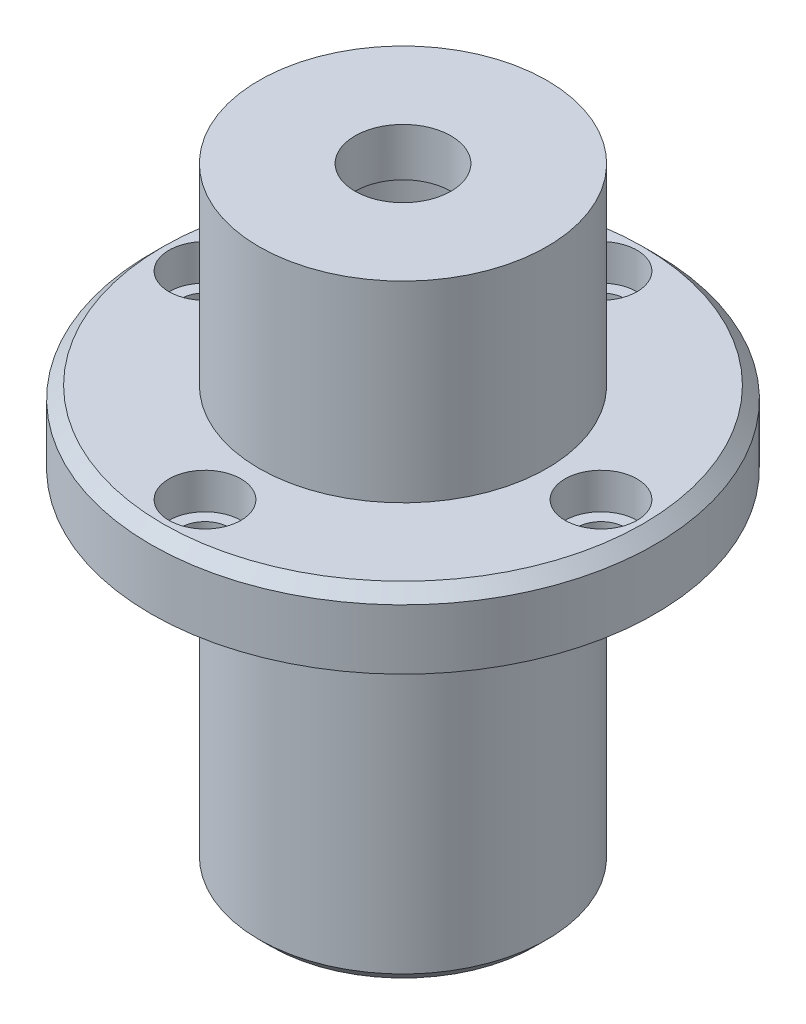
from build123d import *

# Parameters (mm, degrees)
SKETCH1_R           = 12
SKETCH1_R_2         = 4
BOSS_EXTRUDE1_DEPTH = 51
SKETCH2_R           = 8
CUT_EXTRUDE1_DEPTH  = 47
BOSS_EXTRUDE2_START = -6
SKETCH3_R           = 21
SKETCH3_R_2         = 12
BOSS_EXTRUDE2_DEPTH = 6
SKETCH4_R           = 2
CUT_EXTRUDE2_DEPTH  = 6
SKETCH5_R           = 3
CUT_EXTRUDE3_DEPTH  = 3
CIRPATTERN1_COUNT   = 4
CHAMFER1_SIZE       = 1


with BuildPart() as part:
    # Sketch1 → Boss-Extrude1 (new body)
    with BuildSketch(Plane(origin=(0, 0, 0), x_dir=(1, 0, 0), z_dir=(0, 1, 0))):
        with Locations(Location((0, 0, 0), (0, 0, 270))):
            Circle(SKETCH1_R)
        with Locations(Location((0, 0, 0), (0, 0, 270))):
            Circle(SKETCH1_R_2, mode=Mode.SUBTRACT)
    extrude(amount=BOSS_EXTRUDE1_DEPTH)

    # Sketch2 → Cut-Extrude1 (cut)
    with BuildSketch(Plane.XZ):
        with Locations(Location((0, 0, 0), (0, 0, 270))):
            Circle(SKETCH2_R)
    extrude(amount=-CUT_EXTRUDE1_DEPTH, mode=Mode.SUBTRACT)

    # Sketch3 → Boss-Extrude2 (add)
    with BuildSketch(Plane(origin=(0, 35, 0), x_dir=(-1, 0, 0), z_dir=(0, 1, 0)).offset(BOSS_EXTRUDE2_START)):
        with Locations(Location((0, 0, 0), (0, 0, 90))):
            Circle(SKETCH3_R)
        with Locations(Location((0, 0, 0), (0, 0, 90))):
            Circle(SKETCH3_R_2, mode=Mode.SUBTRACT)
    extrude(amount=BOSS_EXTRUDE2_DEPTH)

    # Sketch4 → Cut-Extrude2 (cut)
    with BuildSketch(Plane(origin=(0, 35, 0), x_dir=(1, 0, 0), z_dir=(0, 1, 0))):
        with Locations(Location((0, 16.5, 0), (0, 0, 270))):
            Circle(SKETCH4_R)
    cut_extrude2 = extrude(amount=-CUT_EXTRUDE2_DEPTH, mode=Mode.SUBTRACT)

    # Sketch5 → Cut-Extrude3 (cut)
    with BuildSketch(Plane(origin=(0, 35, 0), x_dir=(1, 0, 0), z_dir=(0, 1, 0))):
        with Locations(Location((0, 16.5, 0), (0, 0, 270))):
            Circle(SKETCH5_R)
    cut_extrude3 = extrude(amount=-CUT_EXTRUDE3_DEPTH, mode=Mode.SUBTRACT)

    # CirPattern1: Cut-Extrude2, Cut-Extrude3 ×4 about axis
    cirpattern1_axis = Axis((0, 0, 0), (0, 1, 0))
    add([cut_extrude2.rotate(cirpattern1_axis, i * 360 / CIRPATTERN1_COUNT) for i in range(1, CIRPATTERN1_COUNT)], mode=Mode.SUBTRACT)
    add([cut_extrude3.rotate(cirpattern1_axis, i * 360 / CIRPATTERN1_COUNT) for i in range(1, CIRPATTERN1_COUNT)], mode=Mode.SUBTRACT)

    # Chamfer1
    chamfer1_edges = [part.edges().sort_by_distance(p)[0] for p in [
        (0, 35, -21),
        (0, 0, -12),
    ]]
    chamfer(chamfer1_edges, length=CHAMFER1_SIZE)


solid = part.part
